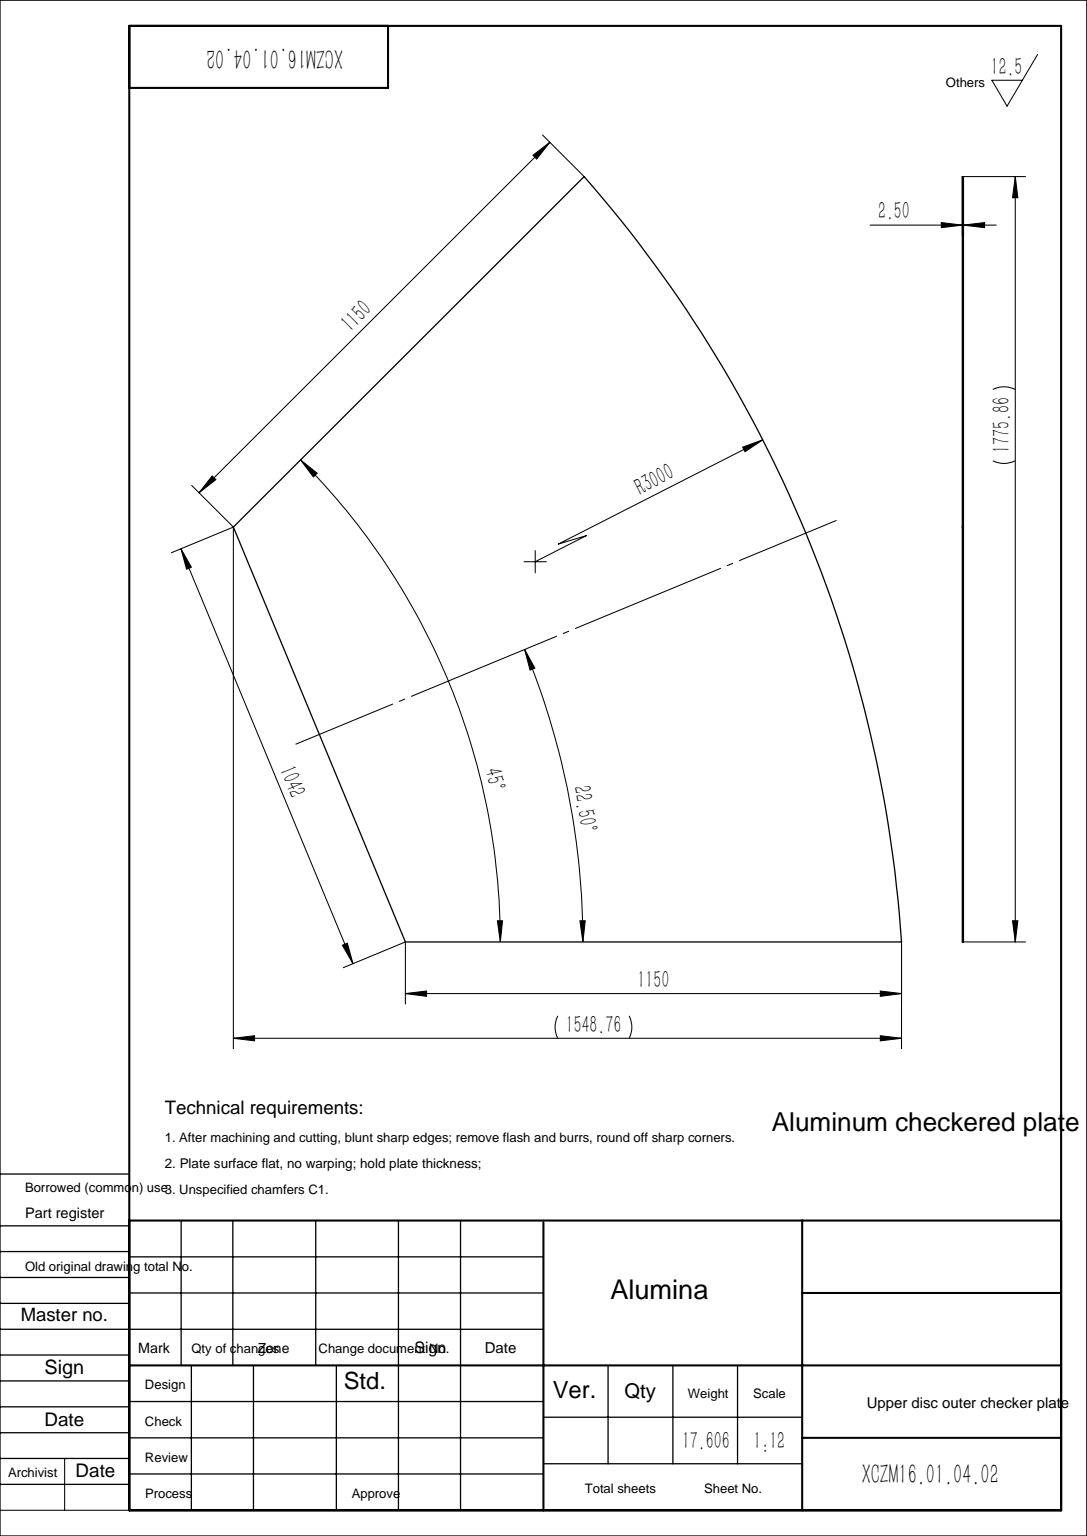
SolidWorks part; units mm, degrees
material "Alumina"
ref_plane "Front Plane" through (0, 0, 0) normal (0, 0, 1) x (1, 0, 0)
ref_plane "Top Plane" through (0, 0, 0) normal (0, 1, 0) x (1, 0, 0)
ref_plane "Right Plane" through (0, 0, 0) normal (1, 0, 0) x (0, 0, -1)
sketch "Sketch2" plane through (0, 0, 0) normal (0, 1, 0) x (1, 0, 0)
  line L0 (0, 0) -> (-398.7561, 962.6825)
  line L1 (0, 0) -> (1150, 0)
  line L2 (414.4167, 1775.8553) -> (-398.7561, 962.6825)
  line L3 (-199.3781, 481.3412) -> (928.287, 948.4354) construction
  arc A0 (1150, 0) -> (414.4167, 1775.8553) centre (-1843.3516, -199.6149) ccw
  dimension "D1" = 1042
  dimension "D3" = 3000
  dimension "D4" = 1150
  dimension "D2" = 45
extrude "Boss-Extrude2" add sketch "Sketch2" along normal blind 2.5
